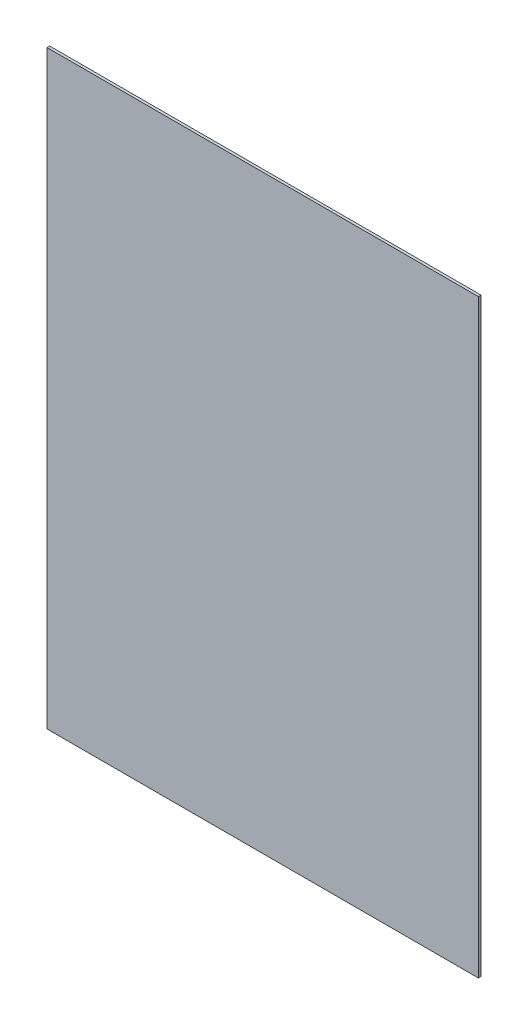
from build123d import *

# Parameters (mm, degrees)
SKETCH_1_W      = 818
SKETCH_1_H      = 1119
EXTRUDE_1_DEPTH = 5


with BuildPart() as part:
    # 草图1 → 凸台-拉伸1 (new body)
    with BuildSketch(Plane.XY):
        Rectangle(SKETCH_1_W, SKETCH_1_H)
    extrude(amount=EXTRUDE_1_DEPTH)


solid = part.part
